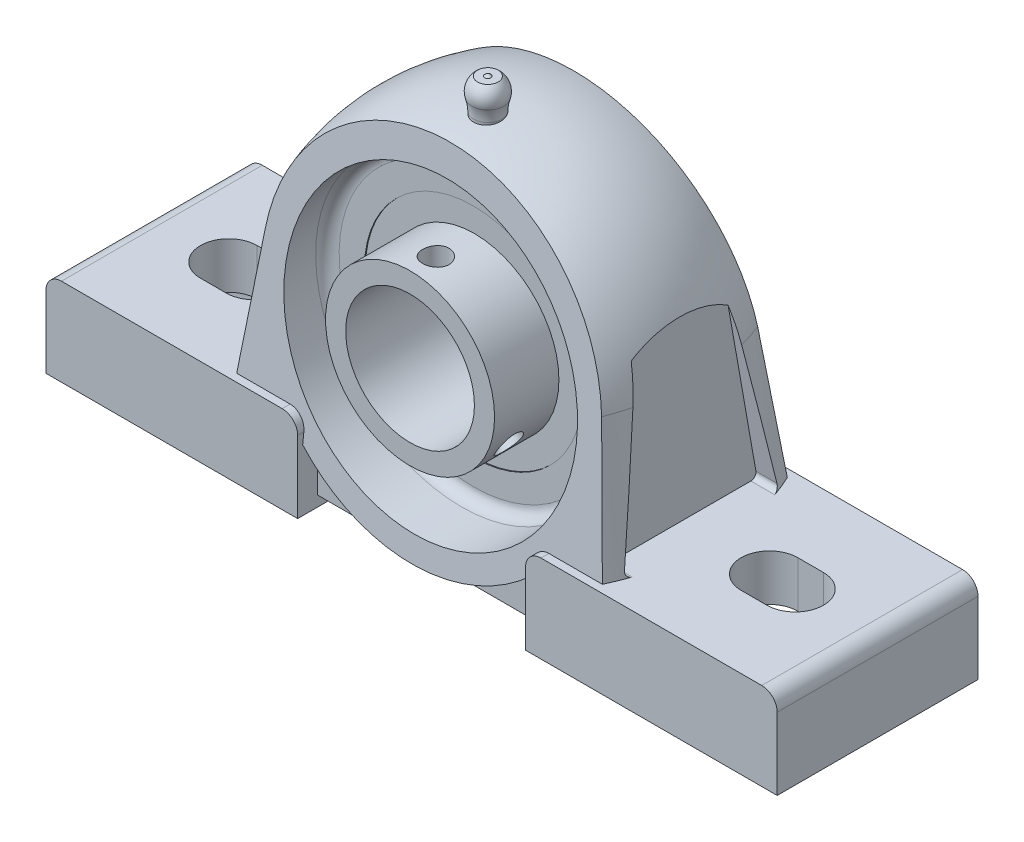
from build123d import *

# Parameters (mm, degrees)
BOSS_EXTRUDE_DEPTH              = 90.55
CUT_EXTRUDE1_DEPTH              = 59.250452667
CUT_EXTRUDE1_DEPTH_BACK         = 59.250452667
SKETCH5_OUTSIDE_W               = 62.184
SKETCH5_OUTSIDE_H               = 95.494
BOSS_EXTRUDE4_REACH             = 64.124
BOSS_EXTRUDE4_DIRECTION_2_REACH = 64.124
BOSS_EXTRUDE1_DEPTH             = 19.5
BOSS_EXTRUDE1_DEPTH_BACK        = 19.5
CUT_EXTRUDE3_DEPTH              = 108.524599994
CUT_EXTRUDE4_DEPTH              = 7.99
CUT_EXTRUDE4_DRAFT              = -1
CUT_EXTRUDE4_PROFILE_2_DEPTH    = 7.99
CUT_EXTRUDE4_PROFILE_2_DRAFT    = -1
CIRPATTERN1_COUNT               = 14
SKETCH14_W                      = 34.1
SKETCH14_H                      = 3.915
SKETCH16_W                      = 2.567
SKETCH16_H                      = 6.115
SKETCH15_W                      = 0.1
SKETCH15_H                      = 5.145
CIRPATTERN2_COUNT               = 2
CIRPATTERN2_ANGLE               = 120
CUT_EXTRUDE5_START              = 32.55942
CUT_EXTRUDE5_DEPTH              = 9.44058
CUT_EXTRUDE6_START              = -42
CUT_EXTRUDE6_DEPTH              = 9.32978


with BuildPart() as part:
    # Sketch1 → Boss-Extrude (new body)
    with BuildSketch(Plane(origin=(0, -34.5, 0), x_dir=(-1, 0, 0), z_dir=(0, 1, 0))):
        with BuildLine():
            Line((-37.693824096, 18.525), (37.693824096, 18.525))
            ThreePointArc((37.693824096, 18.525), (42, 0), (37.693824096, -18.525))
            Line((37.693824096, -18.525), (-37.693824096, -18.525))
            ThreePointArc((-37.693824096, -18.525), (-42, 0), (-37.693824096, 18.525))
        make_face()
    extrude(amount=BOSS_EXTRUDE_DEPTH)

    # Cut-Sweep1: sweep along a path in Sketch3
    with BuildLine(Plane.XY) as cut_sweep1_path:
        Line((-42, -34.5), (-35.386855192, 5.806038205))
        ThreePointArc((-35.386855192, 5.806038205), (0, 35.86), (35.386855192, 5.806038205))
        Line((35.386855192, 5.806038205), (42, -34.5))
    # Sketch2 → Cut-Sweep1 (sweep, cut)
    with BuildSketch(Plane(origin=(0, -34.5, 0), x_dir=(-1, 0, 0), z_dir=(0, 1, 0))):
        with BuildLine():
            Line((-37.693824096, 18.525), (-132.55, 18.525))
            Line((-132.55, 18.525), (-132.55, -18.525))
            Line((-132.55, -18.525), (-37.693824096, -18.525))
            ThreePointArc((-37.693824096, -18.525), (-42, 0), (-37.693824096, 18.525))
        make_face()
    sweep(path=cut_sweep1_path.line, mode=Mode.SUBTRACT)

    # Sketch5 outside → Cut-Extrude1 (cut, two sides: drawn at the far end of the back side and taken through both)
    with BuildSketch(Plane(origin=(0, 0, 0), x_dir=(0, 0, -1), z_dir=(1, 0, 0)).offset(-CUT_EXTRUDE1_DEPTH_BACK)):
        with Locations((0, 0.68)):
            Rectangle(SKETCH5_OUTSIDE_W, SKETCH5_OUTSIDE_H)
        Polygon((11.7, 36.86), (18.525, -24.58), (15.6, -24.58), (15.6, -37.5), (-15.6, -37.5), (-15.6, -24.58), (-18.525, -24.58), (-11.7, 36.86), align=None, mode=Mode.SUBTRACT)
    extrude(amount=CUT_EXTRUDE1_DEPTH + CUT_EXTRUDE1_DEPTH_BACK, mode=Mode.SUBTRACT)

    # Sketch6 → Cut-Revolve2 (revolve, cut)
    with BuildSketch(Plane(origin=(0, 0, 0), x_dir=(0, 0, -1), z_dir=(1, 0, 0)), mode=Mode.PRIVATE) as cut_revolve2_sk:
        with BuildLine():
            Line((-22.455560555, 28.347619048), (-9.777190476, 28.347619048))
            ThreePointArc((-9.777190476, 28.347619048), (-8.166973648, 27.680645399), (-7.5, 26.070428571))
            Line((-7.5, 26.070428571), (-7.5, 24.894778569))
            ThreePointArc((-7.5, 24.894778569), (-6.568548182, 25.156593068), (-5.628, 25.383569804))
            Line((-5.628, 25.383569804), (-5.628, 28.347619048))
            Line((-5.628, 28.347619048), (-3.756, 28.347619048))
            Line((-3.756, 28.347619048), (-3.756, 25.727270823))
            ThreePointArc((-3.756, 25.727270823), (1.917718655, 25.929179608), (7.5, 24.894778569))
            Line((7.5, 24.894778569), (7.5, 26.070428571))
            ThreePointArc((7.5, 26.070428571), (8.166973648, 27.680645399), (9.777190476, 28.347619048))
            Line((9.777190476, 28.347619048), (22.455560555, 28.347619048))
            Line((22.455560555, 28.347619048), (25.604527026, 0))
            Line((25.604527026, 0), (-25.604527026, 0))
            Line((-25.604527026, 0), (-22.455560555, 28.347619048))
        make_face()
    revolve(cut_revolve2_sk.sketch.rotate(Axis((0, 0, 0), (0, 0, -1)), 180), axis=Axis((0, 0, 0), (0, 0, -1)), mode=Mode.SUBTRACT)

    # Sketch11 → Boss-Revolve1 (revolve)
    with BuildSketch(Plane.XY.offset(4.692)):
        with BuildLine():
            Line((0, 34.132633805), (0, 41.86))
            ThreePointArc((0, 41.86), (-0.328456711, 41.790107141), (-0.6, 41.592539267))
            Line((-0.6, 41.592539267), (-2, 41.592539267))
            ThreePointArc((-2, 41.592539267), (-3.100653507, 40.004684437), (-3.105555556, 38.072665525))
            ThreePointArc((-3.105555556, 38.072665525), (-2.83938828, 36.906746373), (-2.75, 35.714176785))
            Line((-2.75, 35.714176785), (-2.75, 34.132633805))
            Line((-2.75, 34.132633805), (0, 34.132633805))
        make_face()
    revolve(axis=Axis((0, 0, 4.692), (0, 1, 0)))

    # Boss-Extrude4: up to this plane
    boss_extrude4_end = Plane(origin=(-42, 36.86, -11.7), z_dir=(0, 0.11040489392462567, -0.9938866934401991))
    # Sketch9 → Boss-Extrude4 (add, up to the surface)
    with BuildSketch(Plane.XY, mode=Mode.PRIVATE) as boss_extrude4_sk1:
        with BuildLine():
            Line((14.121299716, -24.58), (22.128022684, -24.58))
            ThreePointArc((22.128022684, -24.58), (0, -33.073037174), (-22.128022684, -24.58))
            Line((-22.128022684, -24.58), (-14.121299716, -24.58))
            ThreePointArc((-14.121299716, -24.58), (0, -28.347619048), (14.121299716, -24.58))
        make_face()
    boss_extrude4_tool1 = split(extrude(boss_extrude4_sk1.sketch, amount=-BOSS_EXTRUDE4_REACH, mode=Mode.PRIVATE), bisect_by=boss_extrude4_end, keep=Keep.BOTH, mode=Mode.PRIVATE)
    add(boss_extrude4_tool1.solids().sort_by_distance((0, -28.761341, 0))[0])

    # Boss-Extrude4 direction 2: up to this plane
    boss_extrude4_direction_2_end = Plane(origin=(-42, 36.86, 11.7), z_dir=(0, 0.11040489392462567, 0.9938866934401991))
    # Sketch9 → Boss-Extrude4 direction 2 (add, up to the surface)
    with BuildSketch(Plane.XY, mode=Mode.PRIVATE) as boss_extrude4_direction_2_sk1:
        with BuildLine():
            Line((14.121299716, -24.58), (22.128022684, -24.58))
            ThreePointArc((22.128022684, -24.58), (0, -33.073037174), (-22.128022684, -24.58))
            Line((-22.128022684, -24.58), (-14.121299716, -24.58))
            ThreePointArc((-14.121299716, -24.58), (0, -28.347619048), (14.121299716, -24.58))
        make_face()
    boss_extrude4_direction_2_tool1 = split(extrude(boss_extrude4_direction_2_sk1.sketch, amount=BOSS_EXTRUDE4_DIRECTION_2_REACH, mode=Mode.PRIVATE), bisect_by=boss_extrude4_direction_2_end, keep=Keep.BOTH, mode=Mode.PRIVATE)
    add(boss_extrude4_direction_2_tool1.solids().sort_by_distance((0, -28.761341, 0))[0])

    # Sketch4 → Boss-Extrude1 (add, two sides: drawn at the far end of the back side and taken through both)
    with BuildSketch(Plane.XY.offset(-BOSS_EXTRUDE1_DEPTH_BACK)):
        with BuildLine():
            Line((25.128022684, -19.5), (68, -19.5))
            ThreePointArc((68, -19.5), (70.121320344, -20.378679656), (71, -22.5))
            Line((71, -22.5), (71, -36.5))
            Line((71, -36.5), (22.128022684, -36.5))
            Line((22.128022684, -36.5), (22.128022684, -22.5))
            ThreePointArc((22.128022684, -22.5), (23.00670234, -20.378679656), (25.128022684, -19.5))
        make_face()
        with BuildLine():
            Line((-68, -19.5), (-25.128022684, -19.5))
            ThreePointArc((-25.128022684, -19.5), (-23.00670234, -20.378679656), (-22.128022684, -22.5))
            Line((-22.128022684, -22.5), (-22.128022684, -36.5))
            Line((-22.128022684, -36.5), (-71, -36.5))
            Line((-71, -36.5), (-71, -22.5))
            ThreePointArc((-71, -22.5), (-70.121320344, -20.378679656), (-68, -19.5))
        make_face()
    extrude(amount=BOSS_EXTRUDE1_DEPTH + BOSS_EXTRUDE1_DEPTH_BACK)

    # Sketch7 → Cut-Extrude3 (cut, through all)
    with BuildSketch(Plane.XZ.offset(36.5)):
        with BuildLine():
            Line((-50, 5.5), (-55, 5.5))
            ThreePointArc((-55, 5.5), (-60.5, 0), (-55, -5.5))
            Line((-55, -5.5), (-50, -5.5))
            ThreePointArc((-50, -5.5), (-44.5, 0), (-50, 5.5))
        make_face()
        with BuildLine():
            Line((50, -5.5), (55, -5.5))
            ThreePointArc((55, -5.5), (60.5, 0), (55, 5.5))
            Line((55, 5.5), (50, 5.5))
            ThreePointArc((50, 5.5), (44.5, 0), (50, -5.5))
        make_face()
    extrude(amount=-CUT_EXTRUDE3_DEPTH, mode=Mode.SUBTRACT)


with BuildPart() as cut_extrude4_tool:
    # Sketch10 → Cut-Extrude4 (with draft: the straight prism first)
    with BuildSketch(Plane.XZ.offset(36.5)):
        with BuildLine():
            ThreePointArc((55, -10.73), (55.515492065, -9.485492065), (56.76, -8.97))
            Line((56.76, -8.97), (63.975, -8.97))
            ThreePointArc((63.975, -8.97), (65.219507935, -8.454507935), (65.735, -7.21))
            Line((65.735, -7.21), (65.735, 7.21))
            ThreePointArc((65.735, 7.21), (65.219507935, 8.454507935), (63.975, 8.97))
            Line((63.975, 8.97), (56.76, 8.97))
            ThreePointArc((56.76, 8.97), (55.515492065, 9.485492065), (55, 10.73))
            Line((55, 10.73), (55, 12.475))
            ThreePointArc((55, 12.475), (54.484507935, 13.719507935), (53.24, 14.235))
            Line((53.24, 14.235), (29.153022684, 14.235))
            ThreePointArc((29.153022684, 14.235), (27.908514749, 13.719507935), (27.393022684, 12.475))
            Line((27.393022684, 12.475), (27.393022684, -12.475))
            ThreePointArc((27.393022684, -12.475), (27.908514749, -13.719507935), (29.153022684, -14.235))
            Line((29.153022684, -14.235), (53.24, -14.235))
            ThreePointArc((53.24, -14.235), (54.484507935, -13.719507935), (55, -12.475))
            Line((55, -12.475), (55, -10.73))
        make_face()
    extrude(amount=-CUT_EXTRUDE4_DEPTH)
    # Cut-Extrude4: the draft: its side faces are tilted about the plane it starts from
    cut_extrude4_sides = [cut_extrude4_tool.faces().sort_by_distance(p)[0] for p in [
        (55.515492065, -32.505, -9.485492065),
        (60.3675, -32.505, -8.97),
        (65.219507935, -32.505, -8.454507935),
        (65.735, -32.505, 0),
        (65.219507935, -32.505, 8.454507935),
        (60.3675, -32.505, 8.97),
        (55.515492065, -32.505, 9.485492065),
        (55, -32.505, 11.6025),
        (54.484507935, -32.505, 13.719507935),
        (41.196511342, -32.505, 14.235),
        (27.908514749, -32.505, 13.719507935),
        (27.393022684, -32.505, 0),
        (27.908514749, -32.505, -13.719507935),
        (41.196511342, -32.505, -14.235),
        (54.484507935, -32.505, -13.719507935),
        (55, -32.505, -11.6025),
    ]]
    draft(cut_extrude4_sides, Plane.XZ.offset(36.5), CUT_EXTRUDE4_DRAFT)


with BuildPart() as part_1:
    add(part.part)

    # Cut-Extrude4: cut by cut_extrude4_tool
    add(cut_extrude4_tool.part, mode=Mode.SUBTRACT)


with BuildPart() as cut_extrude4_profile_2_tool:
    # Sketch10 → Cut-Extrude4 profile 2 (with draft: the straight prism first)
    with BuildSketch(Plane.XZ.offset(36.5)):
        with BuildLine():
            Line((-63.975, -8.97), (-56.76, -8.97))
            ThreePointArc((-56.76, -8.97), (-55.515492065, -9.485492065), (-55, -10.73))
            Line((-55, -10.73), (-55, -12.475))
            ThreePointArc((-55, -12.475), (-54.484507935, -13.719507935), (-53.24, -14.235))
            Line((-53.24, -14.235), (-29.153022684, -14.235))
            ThreePointArc((-29.153022684, -14.235), (-27.908514749, -13.719507935), (-27.393022684, -12.475))
            Line((-27.393022684, -12.475), (-27.393022684, 12.475))
            ThreePointArc((-27.393022684, 12.475), (-27.908514749, 13.719507935), (-29.153022684, 14.235))
            Line((-29.153022684, 14.235), (-53.24, 14.235))
            ThreePointArc((-53.24, 14.235), (-54.484507935, 13.719507935), (-55, 12.475))
            Line((-55, 12.475), (-55, 10.73))
            ThreePointArc((-55, 10.73), (-55.515492065, 9.485492065), (-56.76, 8.97))
            Line((-56.76, 8.97), (-63.975, 8.97))
            ThreePointArc((-63.975, 8.97), (-65.219507935, 8.454507935), (-65.735, 7.21))
            Line((-65.735, 7.21), (-65.735, -7.21))
            ThreePointArc((-65.735, -7.21), (-65.219507935, -8.454507935), (-63.975, -8.97))
        make_face()
    extrude(amount=-CUT_EXTRUDE4_PROFILE_2_DEPTH)
    # Cut-Extrude4 profile 2: the draft: its side faces are tilted about the plane it starts from
    cut_extrude4_profile_2_sides = [cut_extrude4_profile_2_tool.faces().sort_by_distance(p)[0] for p in [
        (-54.484507935, -32.505, 13.719507935),
        (-55, -32.505, 11.6025),
        (-55.515492065, -32.505, 9.485492065),
        (-60.3675, -32.505, 8.97),
        (-65.219507935, -32.505, 8.454507935),
        (-65.735, -32.505, 0),
        (-65.219507935, -32.505, -8.454507935),
        (-60.3675, -32.505, -8.97),
        (-55.515492065, -32.505, -9.485492065),
        (-55, -32.505, -11.6025),
        (-54.484507935, -32.505, -13.719507935),
        (-41.196511342, -32.505, -14.235),
        (-27.908514749, -32.505, -13.719507935),
        (-27.393022684, -32.505, 0),
        (-27.908514749, -32.505, 13.719507935),
        (-41.196511342, -32.505, 14.235),
    ]]
    draft(cut_extrude4_profile_2_sides, Plane.XZ.offset(36.5), CUT_EXTRUDE4_PROFILE_2_DRAFT)


with BuildPart() as part_2:
    add(part_1.part)

    # Cut-Extrude4 profile 2: cut by cut_extrude4_profile_2_tool
    add(cut_extrude4_profile_2_tool.part, mode=Mode.SUBTRACT)

    # Sketch12 → Boss-Revolve3 (revolve)
    with BuildSketch(Plane(origin=(0, 0, 0), x_dir=(0, 0, -1), z_dir=(1, 0, 0)), mode=Mode.PRIVATE) as boss_revolve3_sk:
        with BuildLine():
            Line((7.5, 24.914778569), (7.5, 21.16))
            Line((7.5, 21.16), (-7.5, 21.16))
            Line((-7.5, 21.16), (-7.5, 24.914778569))
            ThreePointArc((-7.5, 24.914778569), (0, 26.02), (7.5, 24.914778569))
        make_face()
    revolve(boss_revolve3_sk.sketch.rotate(Axis((0, 0, 0), (0, 0, -1)), 180), axis=Axis((0, 0, 0), (0, 0, -1)))

    # Sketch13 → Boss-Revolve4 (revolve)
    with BuildSketch(Plane(origin=(0, 0, 0), x_dir=(0, 0, -1), z_dir=(1, 0, 0))):
        with BuildLine():
            Line((0, 23.1175), (0, 15.4225))
            ThreePointArc((0, 15.4225), (3.8475, 19.27), (0, 23.1175))
        make_face()
    boss_revolve4 = revolve(axis=Axis((0, 0, 0), (0, 1, 0)))

    # CirPattern1: Boss-Revolve4 ×14 about axis
    cirpattern1_axis = Axis((0, 0, 0), (0, 0, 1))
    for i in range(1, CIRPATTERN1_COUNT):
        add(boss_revolve4.rotate(cirpattern1_axis, i * 360 / CIRPATTERN1_COUNT))

    # Sketch14 → Boss-Revolve5 (revolve)
    with BuildSketch(Plane(origin=(0, 0, 0), x_dir=(0, 0, -1), z_dir=(1, 0, 0)), mode=Mode.PRIVATE) as boss_revolve5_sk:
        with Locations((-2.75, 14.4575)):
            Rectangle(SKETCH14_W, SKETCH14_H)
    revolve(boss_revolve5_sk.sketch.rotate(Axis((0, 0, 0), (0, 0, -1)), 90), axis=Axis((0, 0, 0), (0, 0, -1)))

    # Sketch16 → Cut-Revolve3 (revolve, cut)
    with BuildSketch(Plane(origin=(0, 0, 0), x_dir=(0, 0, -1), z_dir=(1, 0, 0))):
        with Locations((-16.0835, 13.5575)):
            Rectangle(SKETCH16_W, SKETCH16_H)
    cut_revolve3 = revolve(axis=Axis((0, 16.615, 14.8), (0, -1, 0)), mode=Mode.SUBTRACT)

    # Sketch15 → Boss-Revolve6 (revolve)
    with BuildSketch(Plane(origin=(0, 0, 0), x_dir=(0, 0, -1), z_dir=(1, 0, 0)), mode=Mode.PRIVATE) as boss_revolve6_sk:
        with Locations((-7.25, 18.7875)):
            Rectangle(SKETCH15_W, SKETCH15_H)
        with Locations((7.25, 18.7875)):
            Rectangle(SKETCH15_W, SKETCH15_H)
    revolve(boss_revolve6_sk.sketch.rotate(Axis((0, 0, 0), (0, 0, -1)), 180), axis=Axis((0, 0, 0), (0, 0, -1)))

    # CirPattern2: Cut-Revolve3 ×2 about axis
    cirpattern2_axis = Axis((0, 0, -21.702927371), (0, 0, -1))
    for i in range(1, CIRPATTERN2_COUNT):
        add(cut_revolve3.rotate(cirpattern2_axis, i * CIRPATTERN2_ANGLE / (CIRPATTERN2_COUNT - 1)), mode=Mode.SUBTRACT)

    # Sketch 17_2 → Cut-Extrude5 (cut)
    with BuildSketch(Plane(origin=(0, 0, 0), x_dir=(0, 0, -1), z_dir=(1, 0, 0)).offset(CUT_EXTRUDE5_START)):
        with BuildLine():
            Line((5.559878946, 34.132633805), (-5.559878946, 34.132633805))
            Line((-5.559878946, 34.132633805), (-14.809813492, -18.326351822))
            ThreePointArc((-14.809813492, -18.326351822), (-14.591050182, -19.14278761), (-13.825005739, -19.5))
            Line((-13.825005739, -19.5), (13.825005739, -19.5))
            ThreePointArc((13.825005739, -19.5), (14.591050182, -19.14278761), (14.809813492, -18.326351822))
            Line((14.809813492, -18.326351822), (5.559878946, 34.132633805))
        make_face()
    extrude(amount=CUT_EXTRUDE5_DEPTH, mode=Mode.SUBTRACT)

    # Sketch 17_2 2 → Cut-Extrude6 (cut)
    with BuildSketch(Plane(origin=(0, 0, 0), x_dir=(0, 0, -1), z_dir=(1, 0, 0)).offset(CUT_EXTRUDE6_START)):
        with BuildLine():
            Line((5.559878946, 34.132633805), (-5.559878946, 34.132633805))
            Line((-5.559878946, 34.132633805), (-14.809813492, -18.326351822))
            ThreePointArc((-14.809813492, -18.326351822), (-14.591050182, -19.14278761), (-13.825005739, -19.5))
            Line((-13.825005739, -19.5), (13.825005739, -19.5))
            ThreePointArc((13.825005739, -19.5), (14.591050182, -19.14278761), (14.809813492, -18.326351822))
            Line((14.809813492, -18.326351822), (5.559878946, 34.132633805))
        make_face()
    extrude(amount=CUT_EXTRUDE6_DEPTH, mode=Mode.SUBTRACT)


solid = part_2.part
